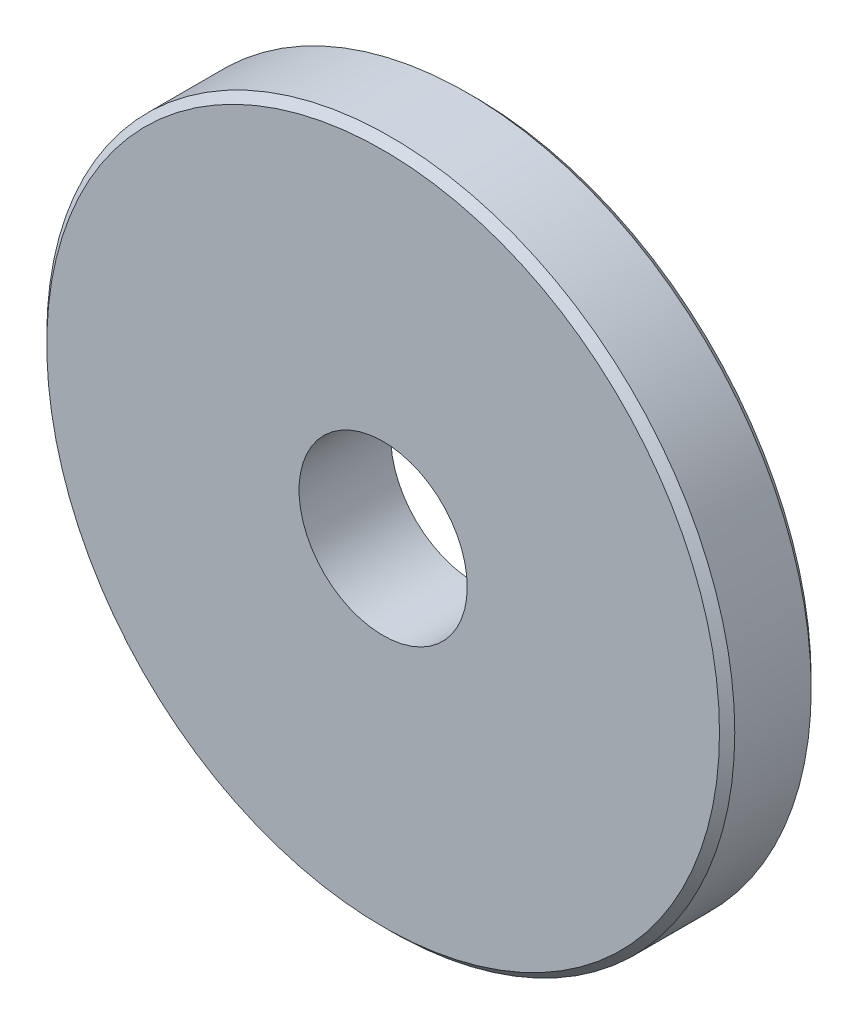
SolidWorks part; units mm, degrees
ref_plane "前视基准面" through (0, 0, 0) normal (0, 0, 1) x (1, 0, 0)
ref_plane "上视基准面" through (0, 0, 0) normal (0, 1, 0) x (1, 0, 0)
ref_plane "右视基准面" through (0, 0, 0) normal (1, 0, 0) x (0, 0, -1)
other "Configuration Table"
sketch "草图1" plane through (0, 0, 0) normal (0, 0, 1) x (1, 0, 0)
  circle A0 centre (0, 0) radius 22.5
  circle A1 centre (0, 0) radius 5.5
  dimension "D1" = 11
  dimension "D2" = 45
extrude "凸台-拉伸1" add sketch "草图1" along normal blind 6
chamfer "倒角1" distance 0.5 angle 45 2 edges at (22.5, 0, 0) (22.5, 0, 6)
